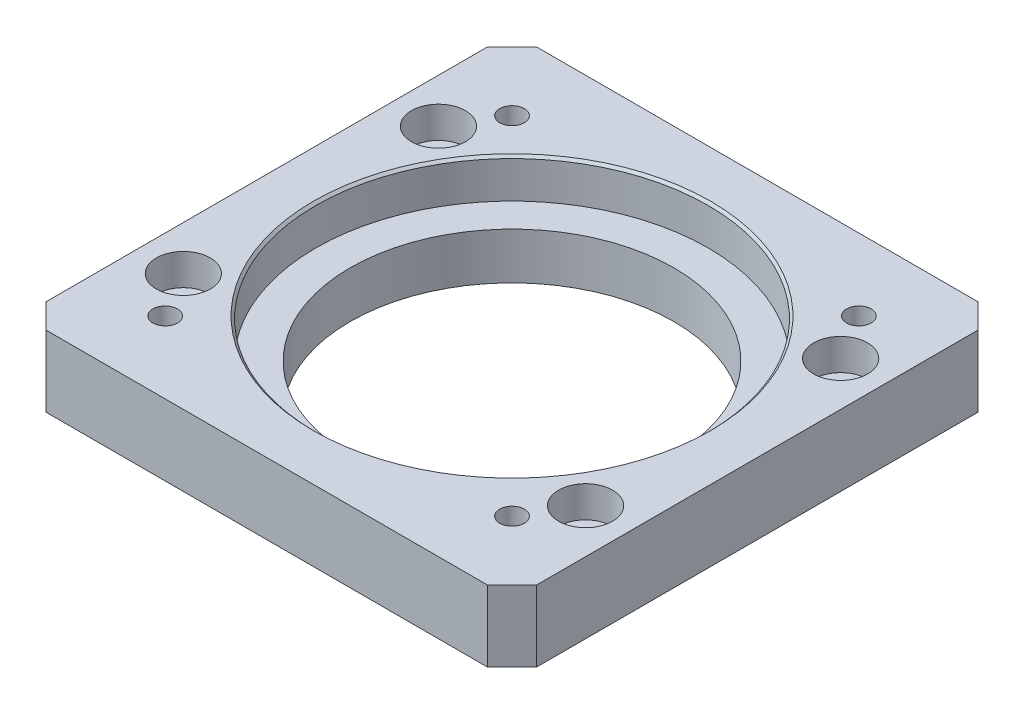
from build123d import *

# Parameters (mm, degrees)
SKETCH_1_W                   = 100
SKETCH_1_H                   = 100
EXTRUDE_1_DEPTH              = 14.5
SKETCH_3_R                   = 36
SKETCH_3_R_2                 = 33
EXTRUDE_2_DEPTH              = 3
SKETCH_4_R                   = 33
CUT_EXTRUDE_1_DEPTH          = 73.182061483
CHAMFER_1_SIZE               = 5
CHAMFER_2_SIZE               = 0.5
SKETCH_10_R                  = 40
CUT_EXTRUDE_3_DEPTH          = 8
HOLE_WIZARD_M6_1_D           = 5
HOLE_WIZARD_M6_1_DEPTH       = 15
HOLE_WIZARD_M6_1_TIP         = 1.502151548
HOLE_WIZARD_M6_2_D           = 6.6
HOLE_WIZARD_M6_2_CBORE_D     = 11
HOLE_WIZARD_M6_2_CBORE_DEPTH = 6.4
CHAMFER_3_SIZE               = 0.5


with BuildPart() as part:
    # 草图1 → 凸台-拉伸1 (new body)
    with BuildSketch(Plane(origin=(0, 0, 0), x_dir=(1, 0, 0), z_dir=(0, 1, 0))):
        Rectangle(SKETCH_1_W, SKETCH_1_H)
    extrude(amount=EXTRUDE_1_DEPTH)

    # 草图3 → 凸台-拉伸2 (add)
    with BuildSketch(Plane.XZ):
        with Locations(Location((0, 0, 0), (0, 0, 270))):
            Circle(SKETCH_3_R)
        with Locations(Location((0, 0, 0), (0, 0, 270))):
            Circle(SKETCH_3_R_2, mode=Mode.SUBTRACT)
    extrude(amount=EXTRUDE_2_DEPTH)

    # 草图4 → 切除-拉伸1 (cut, through all)
    with BuildSketch(Plane.XZ):
        with Locations(Location((0, 0, 0), (0, 0, 270))):
            Circle(SKETCH_4_R)
    extrude(amount=-CUT_EXTRUDE_1_DEPTH, mode=Mode.SUBTRACT)

    # 倒角1
    chamfer_1_edges = [part.edges().sort_by_distance(p)[0] for p in [
        (50, 7.25, 50),
        (-50, 7.25, 50),
        (-50, 7.25, -50),
        (50, 7.25, -50),
    ]]
    chamfer(chamfer_1_edges, length=CHAMFER_1_SIZE)

    # 倒角2
    chamfer_2_edges = [part.edges().sort_by_distance(p)[0] for p in [
        (0, -3, 36),
    ]]
    chamfer(chamfer_2_edges, length=CHAMFER_2_SIZE)

    # 草图10 → 切除-拉伸3 (cut)
    with BuildSketch(Plane(origin=(0, 14.5, 0), x_dir=(1, 0, 0), z_dir=(0, 1, 0))):
        with Locations(Location((0, 0, 0), (0, 0, 270))):
            Circle(SKETCH_10_R)
    extrude(amount=-CUT_EXTRUDE_3_DEPTH, mode=Mode.SUBTRACT)

    # Hole Wizard M6 _1
    with Locations(Plane(origin=(0, 14.5, 0), x_dir=(1, 0, 0), z_dir=(0, 1, 0))):
        with Locations((-35.355, 35.355), (0, 0), (35.355, 35.355), (-35.355, -35.355), (35.355, -35.355)):
            Hole(HOLE_WIZARD_M6_1_D / 2, depth=HOLE_WIZARD_M6_1_DEPTH)
            with Locations((0, 0, -(HOLE_WIZARD_M6_1_DEPTH + HOLE_WIZARD_M6_1_TIP / 2))):  # 118° drill point
                Cone(0, HOLE_WIZARD_M6_1_D / 2, HOLE_WIZARD_M6_1_TIP, mode=Mode.SUBTRACT)

    # M6 六角凹头螺钉的柱形沉头孔2 (through all)
    with Locations(Plane(origin=(0, 14.5, 0), x_dir=(1, 0, 0), z_dir=(0, 1, 0))):
        with Locations((-41, 26), (0, 0), (41, -26), (41, 26), (-41, -26)):
            CounterBoreHole(HOLE_WIZARD_M6_2_D / 2, HOLE_WIZARD_M6_2_CBORE_D / 2, HOLE_WIZARD_M6_2_CBORE_DEPTH)

    # 倒角3
    chamfer_3_edges = [part.edges().sort_by_distance(p)[0] for p in [
        (0, 14.5, -40),
    ]]
    chamfer(chamfer_3_edges, length=CHAMFER_3_SIZE)


solid = part.part
